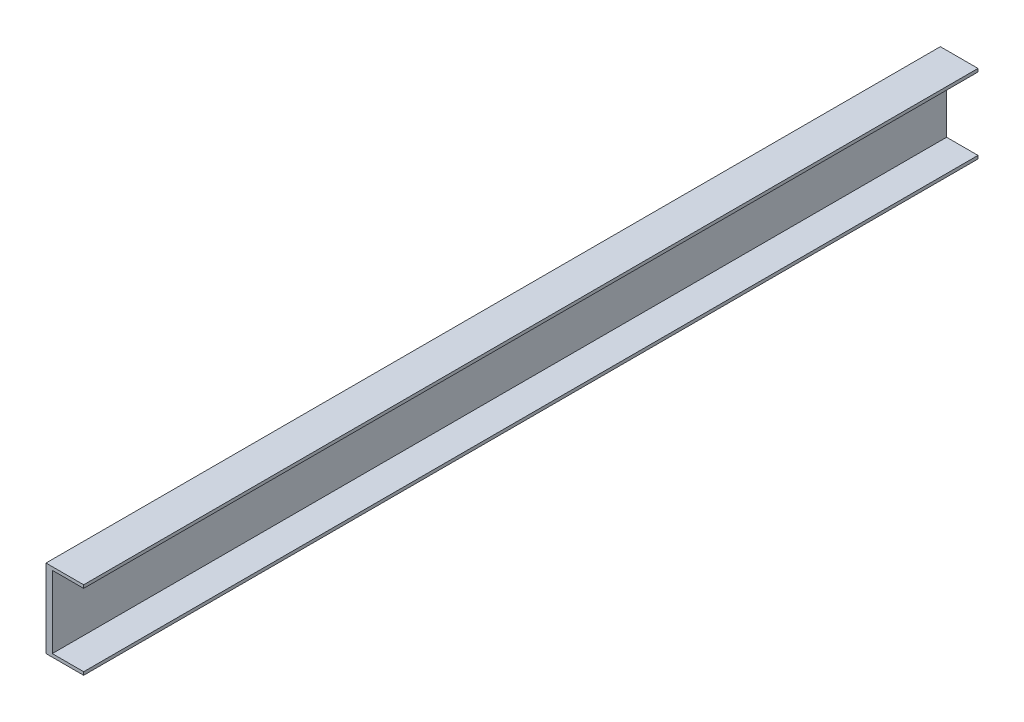
SolidWorks part; units mm, degrees
ref_plane "Front Plane" through (0, 0, 0) normal (0, 0, 1) x (1, 0, 0)
ref_plane "Top Plane" through (0, 0, 0) normal (0, 1, 0) x (1, 0, 0)
ref_plane "Right Plane" through (0, 0, 0) normal (1, 0, 0) x (0, 0, -1)
sketch "Sketch1" plane through (0, 0, 0) normal (0, 0, 1) x (1, 0, 0)
  line L0 (0, 0) -> (-48, 0)
  line L1 (-48, 0) -> (-48, 100)
  line L2 (-48, 100) -> (0, 100)
  line L3 (0, 100) -> (0, 96)
  line L4 (0, 96) -> (-40, 96)
  line L5 (-40, 96) -> (-40, 4)
  line L6 (-40, 4) -> (0, 4)
  line L7 (0, 4) -> (0, 0)
  dimension "D1" = 100
  dimension "D2" = 48
  dimension "D3" = 48
  dimension "D4" = 4
  dimension "D5" = 4
  dimension "D6" = 8
sheet metal parameters "Sheet metal 1" thickness 3 parameters "D1"=3
extrude "Extrude1" add sketch "Sketch1" along normal blind 1140
